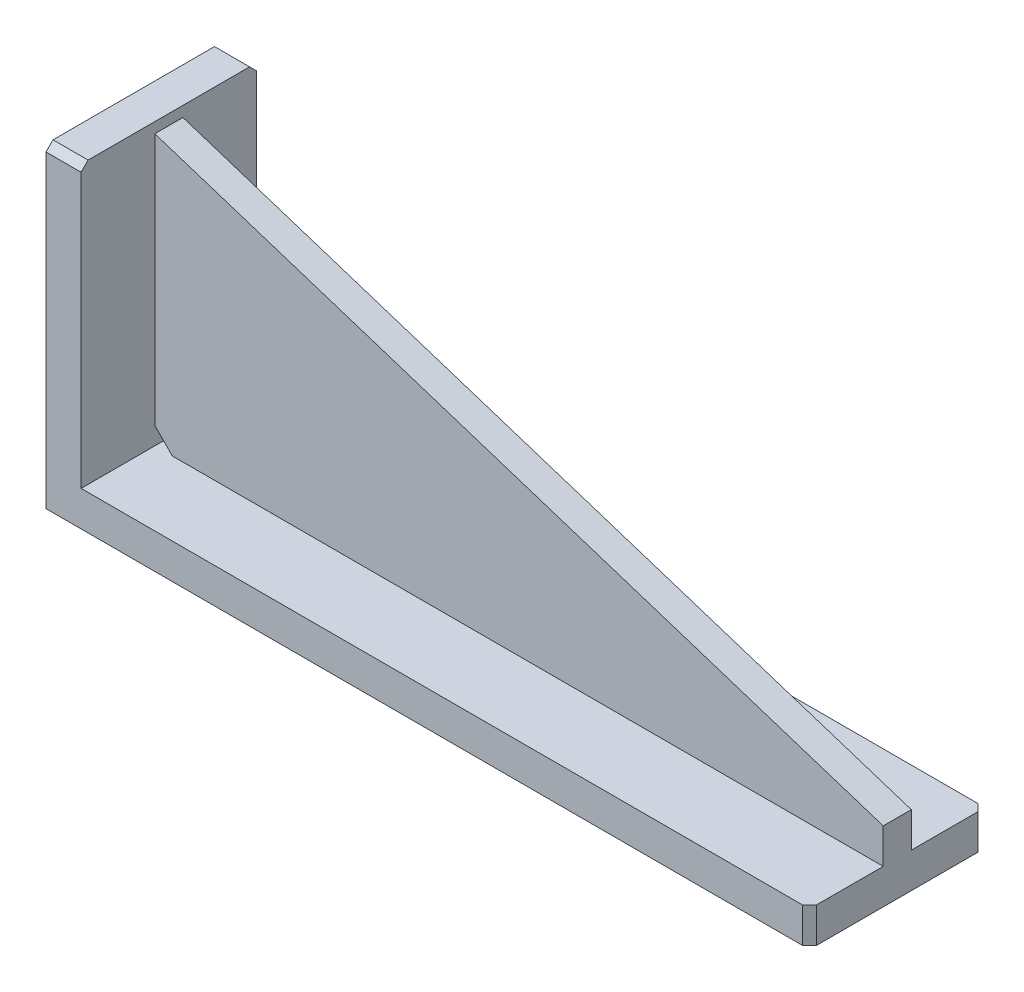
SolidWorks part; units mm, degrees
ref_plane "前视基准面" through (0, 0, 0) normal (0, 0, 1) x (1, 0, 0)
ref_plane "上视基准面" through (0, 0, 0) normal (0, 1, 0) x (1, 0, 0)
ref_plane "右视基准面" through (0, 0, 0) normal (1, 0, 0) x (0, 0, -1)
sketch "草图1" plane through (0, 0, 0) normal (0, 0, 1) x (1, 0, 0)
  line L0 (0, 0) -> (217.5, 0)
  line L1 (217.5, 0) -> (217.5, 10)
  line L2 (217.5, 10) -> (10, 10)
  line L3 (10, 10) -> (10, 90)
  line L4 (10, 90) -> (0, 90)
  line L5 (0, 90) -> (0, 0)
  dimension "D1" = 10
  dimension "D2" = 217.5
  dimension "D3" = 10
  dimension "D4" = 90
extrude "凸台-拉伸1" add sketch "草图1" along normal mid plane 50
sketch "草图2" plane through (0, 0, 0) normal (0, 0, 1) x (1, 0, 0)
  line L0 (10, 87) -> (217.5, 20)
  line L1 (10, 10) -> (10, 90) construction
  line L2 (217.5, 20) -> (217.5, 10)
  line L3 (217.5, 10) -> (10, 10) construction
  line L4 (217.5, 10) -> (15, 10)
  line L5 (15, 10) -> (10, 15)
  line L6 (10, 15) -> (10, 87)
  line L7 (217.5, 0) -> (217.5, 10) construction
  line L8 (10, 90) -> (0, 90) construction
  dimension "D1" = 10
  dimension "D2" = 5
  dimension "D3" = 5
  dimension "D4" = 3
extrude "凸台-拉伸2" add sketch "草图2" along normal mid plane 8
chamfer "倒角1" distance 2 angle 45 4 edges at (217.5, 5, -25) (217.5, 5, 25) (5, 90, 25) (5, 90, -25)
